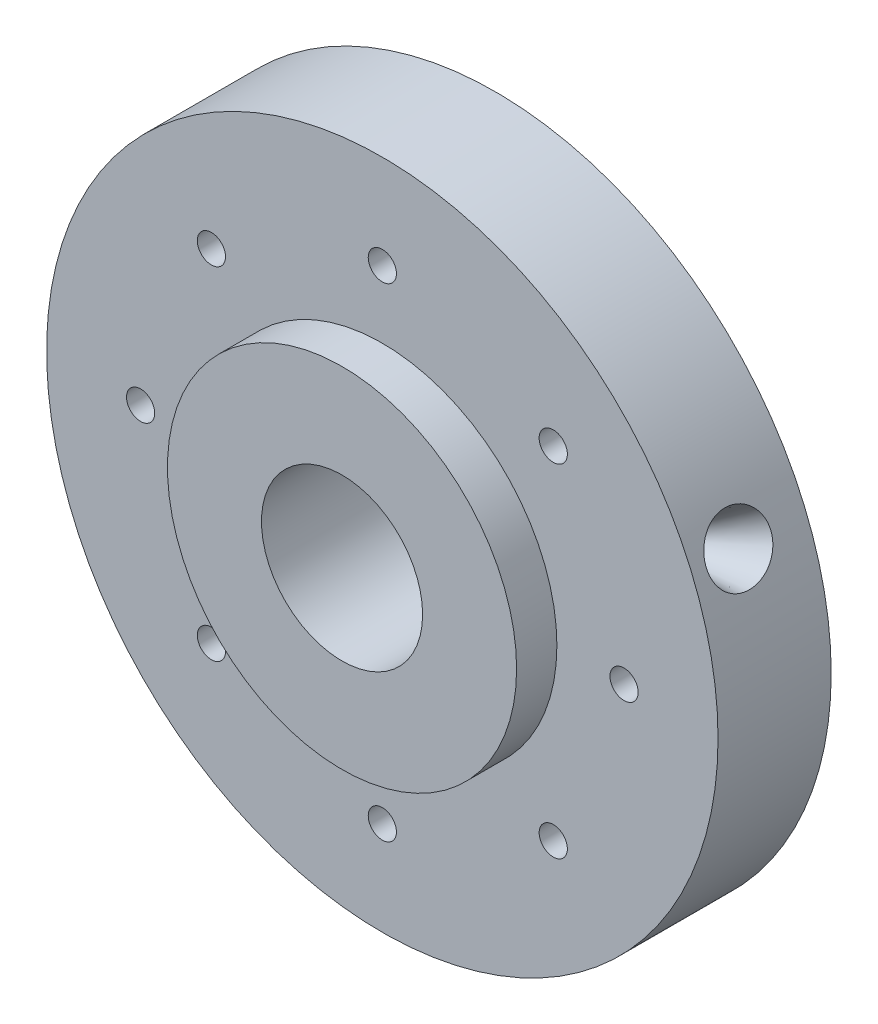
SolidWorks part; units mm, degrees
ref_plane "前视基准面" through (0, 0, 0) normal (0, 0, 1) x (1, 0, 0)
ref_plane "上视基准面" through (0, 0, 0) normal (0, 1, 0) x (1, 0, 0)
ref_plane "右视基准面" through (0, 0, 0) normal (1, 0, 0) x (0, 0, -1)
sketch "草图1" plane through (0, 0, 0) normal (0, 0, 1) x (1, 0, 0)
  circle A0 centre (0, 0) radius 125
  circle A2 centre (0, 90) radius 5.25
  circle A3 centre (63.6396, 63.6396) radius 5.25
  circle A4 centre (90, 0) radius 5.25
  circle A5 centre (63.6396, -63.6396) radius 5.25
  circle A6 centre (0, -90) radius 5.25
  circle A7 centre (-63.6396, -63.6396) radius 5.25
  circle A8 centre (-90, 0) radius 5.25
  circle A9 centre (-63.6396, 63.6396) radius 5.25
  point P22 (0, 0)
  dimension "D1" = 250
  dimension "D3" = 10.5
  dimension "D4" = 8
extrude "凸台-拉伸1" add sketch "草图1" along normal blind 42.13
sketch "草图2" plane through (0, 0, 42.13) normal (0, 0, 1) x (1, 0, 0)
  circle A0 centre (0, 0) radius 65
  dimension "D1" = 130
extrude "凸台-拉伸2" add sketch "草图2" along normal blind 15
sketch "草图3" plane through (0, 0, 57.13) normal (0, 0, 1) x (1, 0, 0)
  circle A0 centre (0, 0) radius 30
  dimension "D1" = 60
extrude "切除-拉伸1" cut sketch "草图3" against normal blind 55
sketch "草图4" plane through (0, 0, 0) normal (0, 1, 0) x (1, 0, 0)
  line L0 (0, 33.3725) -> (0, -104.6961) construction
ref_plane "基准面1" through (0, 0, 0) normal (-0.3827, 0.9239, 0) x (0, 0, 1)
sketch "草图5" plane through (0, 0, 0) normal (-0.3827, 0.9239, 0) x (0, 0, 1)
  line L0 (25, 133.6511) -> (25, -5.6377) construction
  line L1 (0, 125) -> (0, -125) construction
  line L2 (30, 100.5) -> (37.7084, 127.3825)
  line L3 (-33.3725, 0) -> (104.6961, 0) construction
  line L4 (30, 100.5) -> (30, 0)
  line L5 (37.7084, 127.3825) -> (25, 127.3825)
  line L6 (25, 124.9175) -> (25, 0)
  line L7 (25, 0) -> (30, 0)
  line L9 (25, 127.3825) -> (25, 124.9175)
  dimension "D1" = 25
  dimension "D2" = 5
  dimension "D3" = 16
revolve "切除-旋转1" cut sketch "草图5" angle 360 about L0
sketch "草图6" plane through (0, 0, 42.13) normal (0, 0, 1) x (1, 0, 0)
  line L1 (70.1573, 29.0601) -> (-70.1573, -29.0601) construction
  circle A1 centre (43.8843, 18.1775) radius 5
  dimension "D2" = 10
extrude "切除-拉伸2" cut sketch "草图6" against normal blind 50
sketch "草图7" plane through (0, 0, 0) normal (0, 0, -1) x (-1, 0, 0)
  circle A0 centre (0, 90) radius 9
  circle A1 centre (63.6396, 63.6396) radius 9
  circle A2 centre (90, 0) radius 9
  circle A3 centre (63.6396, -63.6396) radius 9
  circle A4 centre (0, -90) radius 9
  circle A5 centre (-63.6396, -63.6396) radius 9
  circle A6 centre (-90, 0) radius 9
  circle A7 centre (-63.6396, 63.6396) radius 9
  point P19 (0, 0)
  dimension "D1" = 18
  dimension "D2" = 8
extrude "切除-拉伸3" cut sketch "草图7" against normal blind 11
